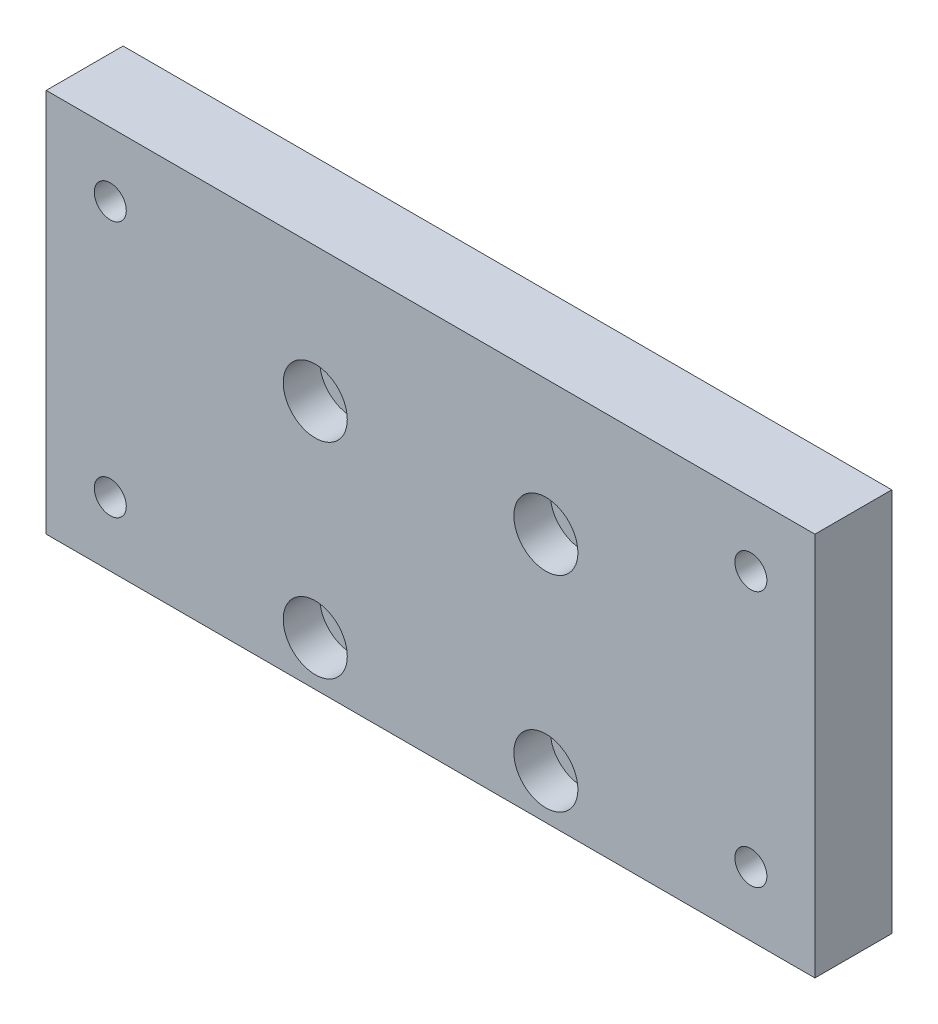
SolidWorks part; units mm, degrees
material "普通碳钢"
ref_plane "Front Plane" through (0, 0, 0) normal (0, 0, 1) x (1, 0, 0)
ref_plane "Top Plane" through (0, 0, 0) normal (0, 1, 0) x (1, 0, 0)
ref_plane "Right Plane" through (0, 0, 0) normal (1, 0, 0) x (0, 0, -1)
sketch "Sketch1" plane through (0, 0, 0) normal (0, 0, 1) x (1, 0, 0)
  line L0 (0, 30) -> (0, -30) construction
  line L1 (-60, -30) -> (60, -30)
  line L2 (-60, -30) -> (-60, 30)
  line L3 (-60, 30) -> (60, 30)
  line L4 (60, -30) -> (60, 30)
  line L5 (-60, -30) -> (60, 30) construction
  line L6 (-60, 30) -> (60, -30) construction
  line L7 (-60, 0) -> (60, 0) construction
  circle A0 centre (-50, 20) radius 1.5
  circle A1 centre (50, 20) radius 1.5
  circle A2 centre (50, -20) radius 1.5
  circle A3 centre (-50, -20) radius 1.5
  point P0 (0, 0)
  dimension "D3" = 3
  dimension "D1" = 120
  dimension "D2" = 60
  dimension "D4" = 40
  dimension "D5" = 100
  dimension "D6" = 50
  dimension "D7" = 20
extrude "Boss-Extrude1" add sketch "Sketch1" along normal blind 12
hole_wizard "Hole Size (per hex socket screw type)1" positions "3DSketch1" profile "Sketch2" counterbore size "M5" standard "GB"
sketch3d "3DSketch1"
  line L0 (0, 30, 12) -> (0, -30, 12) construction
  line L1 (60, 30, 12) -> (-60, 30, 12) construction
  line L2 (-60, -30, 12) -> (60, -30, 12) construction
  line L4 (-18, 9, 12) -> (18, 9, 12) construction
  point P0 (-18, 9, 12)
  point P2 (18, 9, 12)
  point P4 (-18, -23, 12)
  point P6 (18, -23, 12)
  dimension "D1" = 36
  dimension "D2" = 36
  dimension "D3" = 32
  dimension "D4" = 32
  dimension "D5" = 18
  dimension "D6" = 21
  dimension "D7" = 18
sketch "Sketch2" plane through (-18, 9, 12) normal (1, 0, 0) x (0, -1, 0)
  line L0 (0, 0) -> (0, 19.6524)
  line L1 (0, 19.6524) -> (2.75, 18)
  line L2 (2.75, 18) -> (2.75, 5.7)
  line L3 (2.75, 5.7) -> (5, 5.7)
  line L4 (5, 5.7) -> (5, 0)
  line L5 (5, 0) -> (0, 0)
  line L10 (0, 19.6524) -> (-2.75, 18) construction
  line L11 (0, -6.35) -> (0, 107.95) construction
  dimension "孔直径" = 5.5
  dimension "孔深度" = 18
  dimension "柱形沉头孔直径" = 10
  dimension "柱形沉头孔深度" = 5.7
  dimension "导头角度" = 118
hole_wizard "M6 Tapped Hole1" positions "Sketch3" profile "Sketch4" tap size "M6" standard "GB"
sketch "Sketch3" plane through (0, 0, 12) normal (0, 0, 1) x (1, 0, 0)
  point P0 (-50, 20)
  point P3 (-50, -20)
  point P6 (50, -20)
  point P9 (50, 20)
sketch "Sketch4" plane through (-50, 20, 12) normal (1, 0, 0) x (0, -1, 0)
  line L0 (0, 0) -> (0, 16.5022)
  line L1 (0, 16.5022) -> (2.5, 15)
  line L2 (2.5, 15) -> (2.5, 0)
  line L5 (2.5, 0) -> (0, 0)
  line L10 (0, 16.5022) -> (-2.5, 15) construction
  line L11 (0, -6.35) -> (0, 107.95) construction
  dimension "螺纹孔钻头直径" = 5
  dimension "螺纹孔钻头深度" = 15
  dimension "导头角度" = 118
cosmetic thread "Cosmetic Thread1" parameters "D1"=12, "D2"=6
cosmetic thread "Cosmetic Thread2" parameters "D1"=12, "D2"=6
cosmetic thread "Cosmetic Thread3" parameters "D1"=12, "D2"=6
cosmetic thread "Cosmetic Thread4" parameters "D1"=12, "D2"=6
